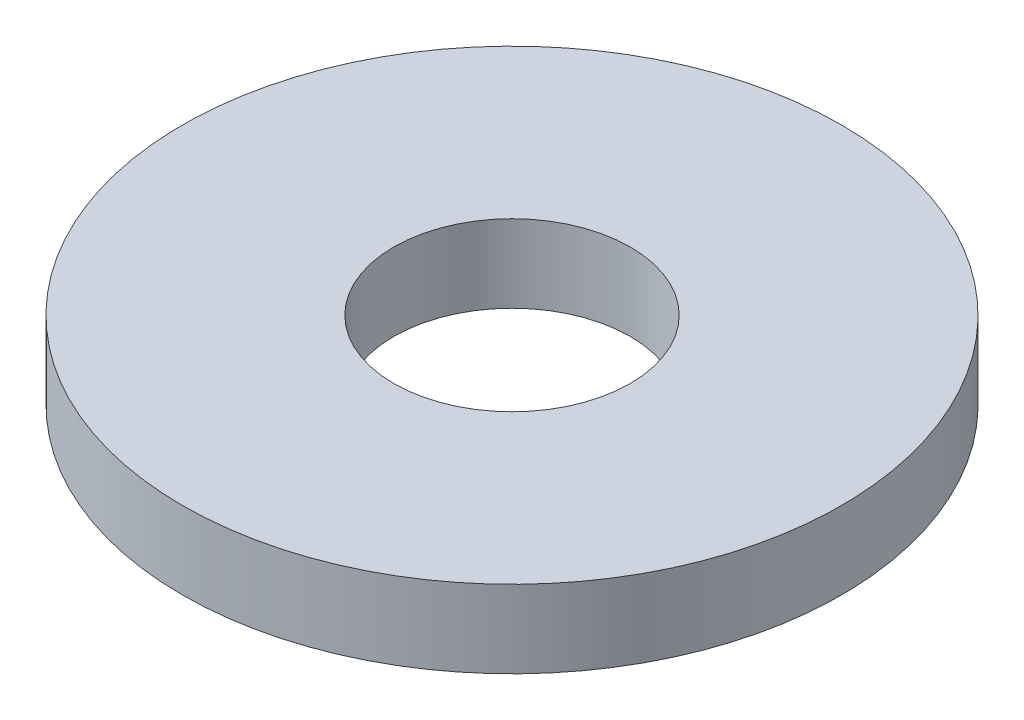
SolidWorks part; units mm, degrees
ref_plane "Front Plane" through (0, 0, 0) normal (0, 0, 1) x (1, 0, 0)
ref_plane "Top Plane" through (0, 0, 0) normal (0, 1, 0) x (1, 0, 0)
ref_plane "Right Plane" through (0, 0, 0) normal (1, 0, 0) x (0, 0, -1)
sketch "Sketch1" plane through (0, 0, 0) normal (0, 1, 0) x (1, 0, 0)
  circle A0 centre (0, 0) radius 4.25
  circle A1 centre (0, 0) radius 1.525
  dimension "D1" = 8.5
  dimension "D2" = 3.05
extrude "Boss-Extrude1" add sketch "Sketch1" along normal blind 1
